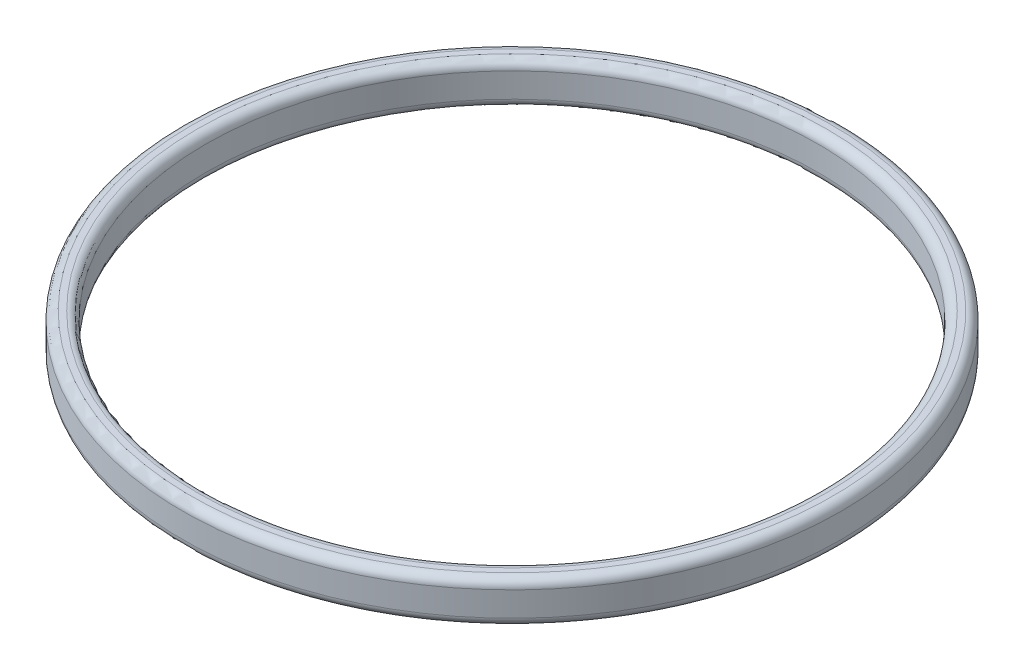
from build123d import *


with BuildPart() as part:
    # 草图1 → 旋转1 (revolve)
    with BuildSketch(Plane.XY):
        with BuildLine():
            Line((-36.2806, 5.587), (-36.973, 5.587))
            ThreePointArc((-36.973, 5.587), (-37.680106781, 5.879893219), (-37.973, 6.587))
            Line((-37.973, 6.587), (-37.973, 9.413))
            ThreePointArc((-37.973, 9.413), (-37.680106781, 10.120106781), (-36.973, 10.413))
            Line((-36.973, 10.413), (-36.2806, 10.413))
            ThreePointArc((-36.2806, 10.413), (-35.573493219, 10.120106781), (-35.2806, 9.413))
            Line((-35.2806, 9.413), (-35.2806, 6.587))
            ThreePointArc((-35.2806, 6.587), (-35.573493219, 5.879893219), (-36.2806, 5.587))
        make_face()
    revolve(axis=Axis((0, 27, 0), (0, -1, 0)))


solid = part.part
